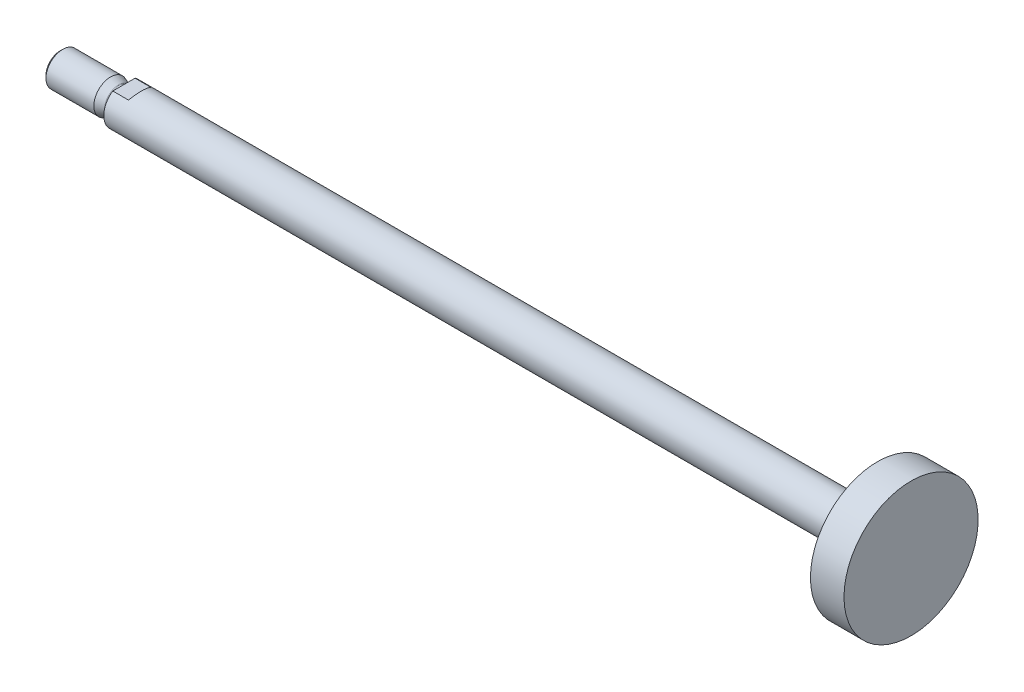
SolidWorks part; units mm, degrees
ref_plane "前视基准面" through (0, 0, 0) normal (0, 0, 1) x (1, 0, 0)
ref_plane "上视基准面" through (0, 0, 0) normal (0, 1, 0) x (1, 0, 0)
ref_plane "右视基准面" through (0, 0, 0) normal (1, 0, 0) x (0, 0, -1)
ref_plane "基准面4" through (0, 0, 0) normal (0, 0, -1) x (-1, 0, 0)
sketch "草图1" plane through (0, 0, 0) normal (0, 0, -1) x (-1, 0, 0)
  line L0 (-228.6, 20) -> (-228.6, 0)
  line L1 (-228.6, 0) -> (-218.6, 0)
  line L2 (-218.6, 0) -> (-218.6, 20)
  line L3 (-218.6, 20) -> (-228.6, 20)
  line L4 (-228.6, 0) -> (-218.6, 0) construction
revolve "旋转1" add sketch "草图1" angle 360 about L4
sketch "草图2" plane through (218.6, 0, 0) normal (-1, 0, 0) x (0, 0, 1)
  circle A0 centre (0, 0) radius 6
extrude "凸台-拉伸1" add sketch "草图2" along normal blind 224.7
sketch "草图3" plane through (-6.1, 0, 0) normal (-1, 0, 0) x (0, 0, 1)
  line L0 (-3.3166, 5) -> (3.3166, 5)
  arc A0 (3.3166, 5) -> (-3.3166, 5) centre (0, 0) ccw
extrude "切除-拉伸1" cut sketch "草图3" against normal blind 4.7
sketch "草图4" plane through (-6.1, 0, 0) normal (-1, 0, 0) x (0, 0, 1)
  line L0 (3.3166, -5) -> (-3.3166, -5)
  arc A0 (-3.3166, -5) -> (3.3166, -5) centre (0, 0) ccw
extrude "切除-拉伸2" cut sketch "草图4" against normal blind 4.7
sketch "草图5" plane through (-6.1, 0, 0) normal (-1, 0, 0) x (0, 0, 1)
  circle A0 centre (0, 0) radius 4.1
extrude "凸台-拉伸2" add sketch "草图5" along normal blind 1.5
sketch "草图6" plane through (-7.6, 0, 0) normal (-1, 0, 0) x (0, 0, 1)
  circle A0 centre (0, 0) radius 4.1
extrude "凸台-拉伸3" add sketch "草图6" along normal blind 2.4727 draft 20 draft outward yes
sketch "草图7" plane through (-10.0727, 0, 0) normal (-1, 0, 0) x (0, 0, 1)
  circle A0 centre (0, 0) radius 5
extrude "凸台-拉伸4" add sketch "草图7" along normal blind 15.0273
draft "拔模1" type of draft neutral plane draft angle 30 faces to draft 1 face at (-1.4, -5.5, 0) neutral plane through (-1.4, -5, 3.3166) neutral plane normal (0, -1, 0) parameters "D1"=30
draft "拔模2" type of draft neutral plane draft angle 30 faces to draft 1 face at (-1.4, 5.5, 0) neutral plane through (-1.4, 5, -3.3166) neutral plane normal (0, 1, 0) parameters "D1"=30
chamfer "倒角1" distance 0.767 angle 45 1 edges at (-25.1, 0, 5)
fillet "圆角1" radius 0.6 2 edges at (-6.1, 0, 4.1) (-7.6, 0, 4.1)
